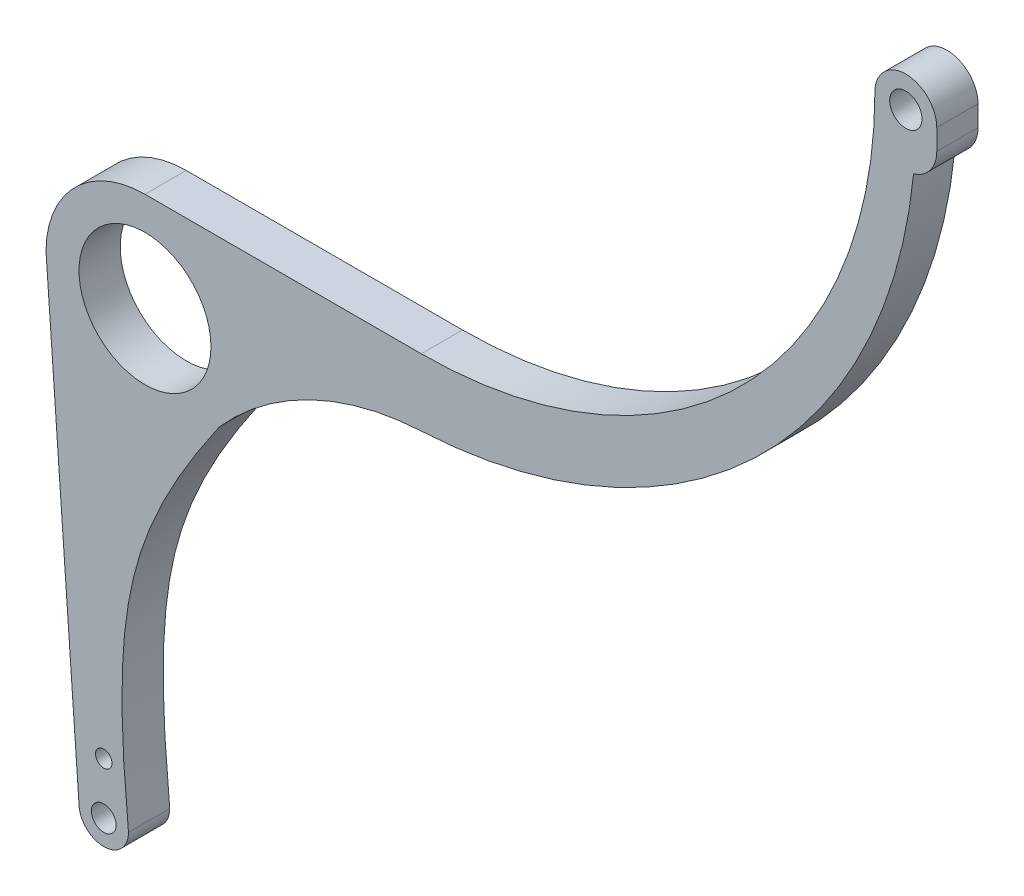
from build123d import *

# Parameters (mm, degrees)
SKETCH_1_R      = 3
SKETCH_1_R_2    = 16
SKETCH_1_R_3    = 3.91899873
SKETCH_1_R_4    = 2
EXTRUDE_1_DEPTH = 10


with BuildPart() as part:
    # 草图1 → 凸台-拉伸1 (new body)
    with BuildSketch(Plane.XY):
        with BuildLine():
            Line((-14, 112), (-6, 0))
            ThreePointArc((-6, 0), (0, -6), (6, 0))
            add(Edge.make_bspline(
                [(6, 0), (1.588652615, 45.680929706), (5.604102499, 63.643200211), (28.004797731, 96.13093391)],
                knots=[0, 0, 0, 0, 0.788155359, 0.788155359, 0.788155359, 0.788155359], degree=3))
            ThreePointArc((28.004797731, 96.13093391), (50.113637924, 112.900750568), (77, 119.767416406))
            ThreePointArc((77, 119.767416406), (157.787149523, 154.485384951), (196.379869136, 233.494896157))
            ThreePointArc((196.379869136, 233.494896157), (200.439238403, 236.311917913), (202, 241))
            Line((202, 241), (202, 246))
            ThreePointArc((202, 246), (194.5, 253.5), (187, 246))
            ThreePointArc((187, 246), (154.781745931, 168.218254069), (77, 136))
            Line((77, 136), (10, 136))
            ThreePointArc((10, 136), (-6.970562748, 128.970562748), (-14, 112))
        make_face()
        Circle(SKETCH_1_R, mode=Mode.SUBTRACT)
        with Locations((10, 112)):
            Circle(SKETCH_1_R_2, mode=Mode.SUBTRACT)
        with Locations((194.5, 246)):
            Circle(SKETCH_1_R_3, mode=Mode.SUBTRACT)
        with Locations((0, 12.5)):
            Circle(SKETCH_1_R_4, mode=Mode.SUBTRACT)
    extrude(amount=EXTRUDE_1_DEPTH)


solid = part.part
